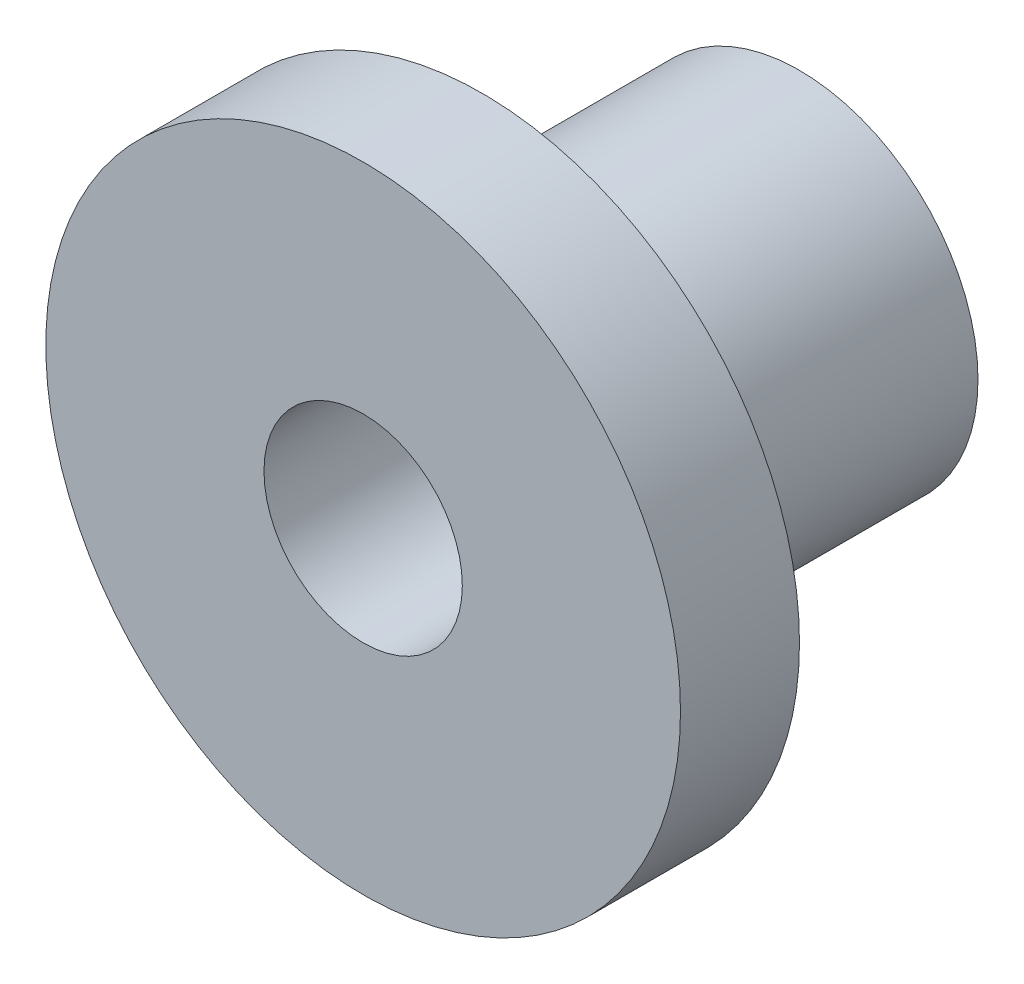
from build123d import *

# Parameters (mm, degrees)
SKETCH1_R           = 22.5
BOSS_EXTRUDE1_DEPTH = 40
SKETCH2_R           = 40
BOSS_EXTRUDE2_DEPTH = 15
SKETCH3_R           = 12.5
CUT_EXTRUDE1_DEPTH  = 97


with BuildPart() as part:
    # Sketch1 → Boss-Extrude1 (new body)
    with BuildSketch(Plane.XY):
        Circle(SKETCH1_R)
    extrude(amount=BOSS_EXTRUDE1_DEPTH)

    # Sketch2 → Boss-Extrude2 (add)
    with BuildSketch(Plane.XY.offset(40)):
        Circle(SKETCH2_R)
    extrude(amount=BOSS_EXTRUDE2_DEPTH)

    # Sketch3 → Cut-Extrude1 (cut)
    with BuildSketch(Plane(origin=(0, 0, 0), x_dir=(-1, 0, 0), z_dir=(0, 0, -1))):
        Circle(SKETCH3_R)
    extrude(amount=-CUT_EXTRUDE1_DEPTH, mode=Mode.SUBTRACT)


solid = part.part
